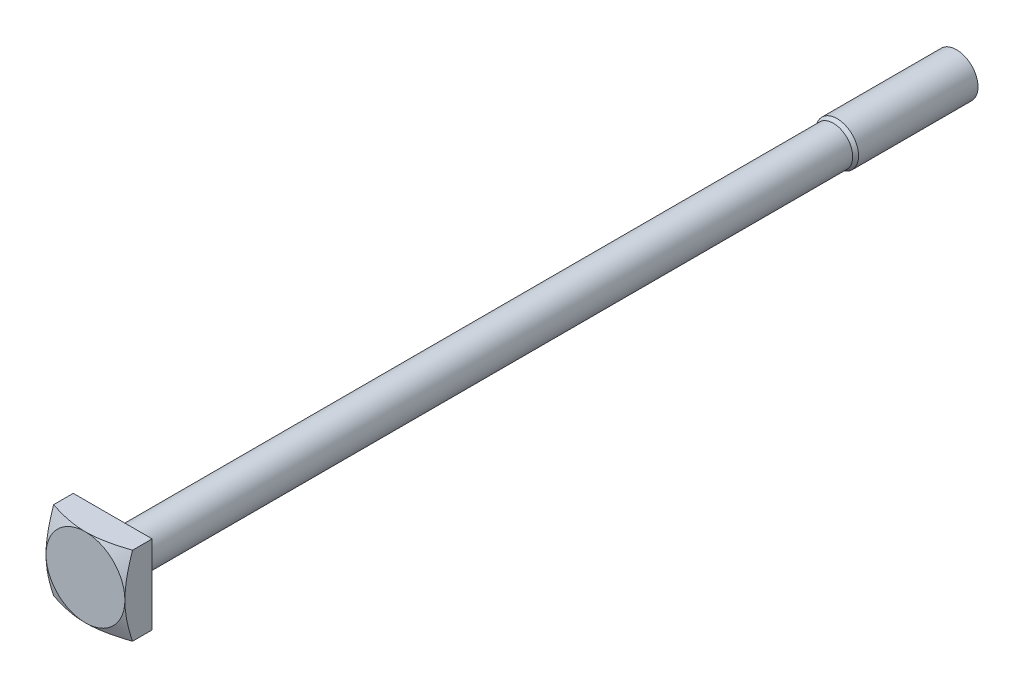
from build123d import *

# Parameters (mm, degrees)
SKETCH1_W          = 55
SKETCH1_H          = 55
BASE_EXTRUDE_DEPTH = 19
SKETCH4_OUTSIDE_W  = 262.948
SKETCH4_OUTSIDE_H  = 262.948
SKETCH4_OUTSIDE_R  = 27.5
CUT_EXTRUDE1_DEPTH = 44.283946216
CUT_EXTRUDE1_DRAFT = -65
FILLET1_R          = 1


with BuildPart() as part:
    # Sketch1 → Base-Extrude (new body)
    with BuildSketch(Plane.XY):
        Rectangle(SKETCH1_W, SKETCH1_H)
    extrude(amount=BASE_EXTRUDE_DEPTH)


with BuildPart() as cut_extrude1_tool:
    # Sketch4 outside → Cut-Extrude1 (with draft: the straight prism first)
    with BuildSketch(Plane.XY.offset(19)):
        Rectangle(SKETCH4_OUTSIDE_W, SKETCH4_OUTSIDE_H)
        Circle(SKETCH4_OUTSIDE_R, mode=Mode.SUBTRACT)
    extrude(amount=-CUT_EXTRUDE1_DEPTH)
    # Cut-Extrude1: the draft: its side faces are tilted about the plane it starts from
    cut_extrude1_sides = [cut_extrude1_tool.faces().sort_by_distance(p)[0] for p in [
        (0, -131.474, -3.141973108),
        (131.474, 0, -3.141973108),
        (0, 131.474, -3.141973108),
        (-131.474, 0, -3.141973108),
        (-27.5, 0, -3.141973108),
    ]]
    draft(cut_extrude1_sides, Plane.XY.offset(19), CUT_EXTRUDE1_DRAFT)


with BuildPart() as part_1:
    add(part.part)

    # Cut-Extrude1: cut by cut_extrude1_tool
    add(cut_extrude1_tool.part, mode=Mode.SUBTRACT)

    # Sketch2 → Boss-Revolve1 (revolve)
    with BuildSketch(Plane(origin=(0, 0, 0), x_dir=(1, 0, 0), z_dir=(0, 1, 0)), mode=Mode.PRIVATE) as boss_revolve1_sk:
        Polygon((0, 0), (13.5, 0), (13.5, 502.401923789), (15, 505), (15, 590), (0, 590), align=None)
    revolve(boss_revolve1_sk.sketch.rotate(Axis((0, 0, -590), (0, 0, 1)), 180), axis=Axis((0, 0, -590), (0, 0, 1)))

    # Fillet1
    fillet1_edges = [part_1.edges().sort_by_distance(p)[0] for p in [
        (13.5, 0, 0),
    ]]
    fillet(fillet1_edges, radius=FILLET1_R)

    # Sketch3 → Cut-Revolve1 (revolve, cut)
    with BuildSketch(Plane(origin=(0, 0, 0), x_dir=(1, 0, 0), z_dir=(0, 1, 0))):
        Polygon((11.969, 590), (15, 591.749948666), (15, 588.250051334), align=None)
    revolve(axis=Axis((0, 0, 0), (0, 0, -1)), mode=Mode.SUBTRACT)


solid = part_1.part
